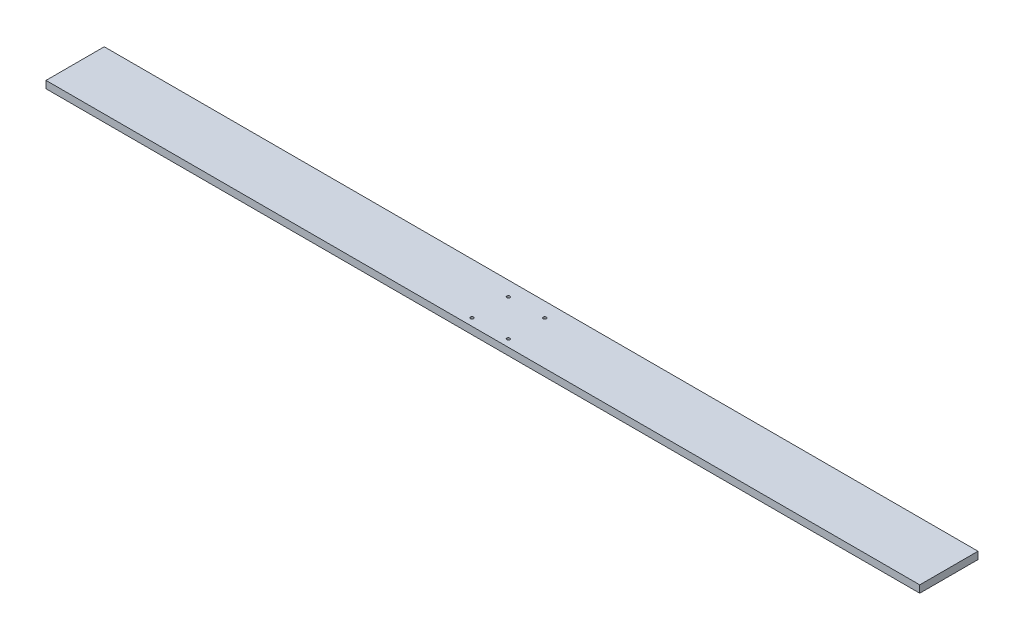
from build123d import *

# Parameters (mm, degrees)
SKETCH_2_W          = 1200
SKETCH_2_H          = 80
EXTRUDE_1_DEPTH     = 5
SKETCH_4_R          = 2.1
CUT_EXTRUDE_1_DEPTH = 26


with BuildPart() as part:
    # 草图2 → 凸台-拉伸1 (new, symmetric)
    with BuildSketch(Plane(origin=(0, 0, 0), x_dir=(1, 0, 0), z_dir=(0, 1, 0))):
        Rectangle(SKETCH_2_W, SKETCH_2_H)
    extrude(amount=EXTRUDE_1_DEPTH, both=True)

    # 草图4 → 切除-拉伸1 (cut)
    with BuildSketch(Plane(origin=(0, 5, 0), x_dir=(1, 0, 0), z_dir=(0, 1, 0))):
        with Locations(Location((-25, 20, 0), (0, 0, 270))):
            Circle(SKETCH_4_R)
        with Locations(Location((25, 20, 0), (0, 0, 270))):
            Circle(SKETCH_4_R)
        with Locations(Location((25, -30, 0), (0, 0, 270))):
            Circle(SKETCH_4_R)
        with Locations(Location((-25, -30, 0), (0, 0, 270))):
            Circle(SKETCH_4_R)
    extrude(amount=-CUT_EXTRUDE_1_DEPTH, mode=Mode.SUBTRACT)


solid = part.part
